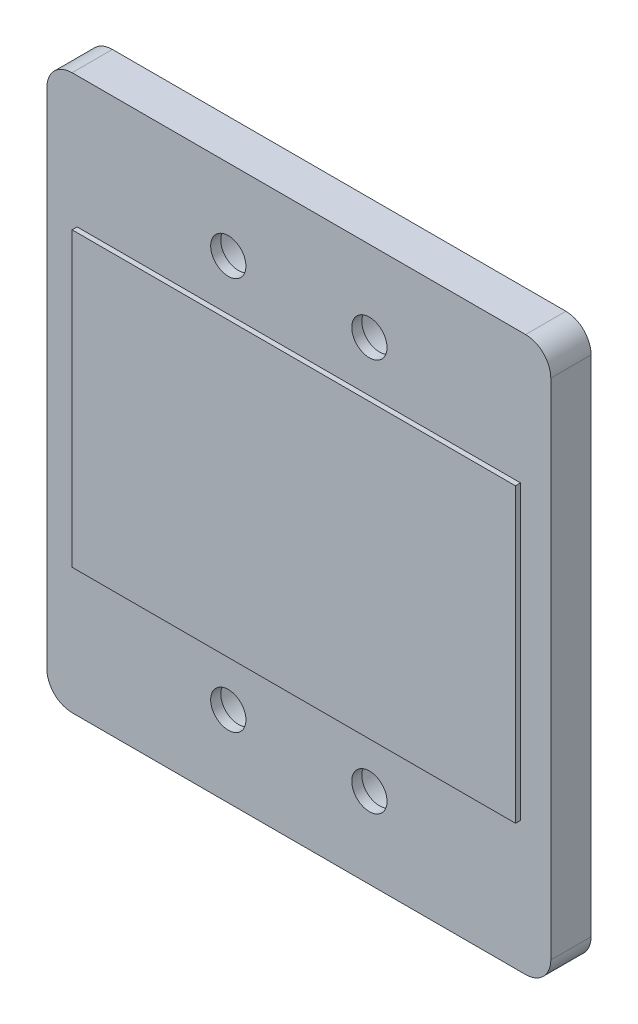
from build123d import *

# Parameters (mm, degrees)
BOSS_EXTRUDE1_DEPTH = 8
SKETCH2_W           = 88
SKETCH2_H           = 58
BOSS_EXTRUDE2_DEPTH = 1
SKETCH4_R           = 6
CUT_EXTRUDE1_DEPTH  = 6
SKETCH5_R           = 3.5
CUT_EXTRUDE2_DEPTH  = 6


with BuildPart() as part:
    # Sketch1 → Boss-Extrude1 (new body)
    with BuildSketch(Plane.XY):
        with BuildLine():
            Line((-45, -55), (45, -55))
            ThreePointArc((45, -55), (48.535533906, -53.535533906), (50, -50))
            Line((50, -50), (50, 50))
            ThreePointArc((50, 50), (48.535533906, 53.535533906), (45, 55))
            Line((45, 55), (-45, 55))
            ThreePointArc((-45, 55), (-48.535533906, 53.535533906), (-50, 50))
            Line((-50, 50), (-50, -50))
            ThreePointArc((-50, -50), (-48.535533906, -53.535533906), (-45, -55))
        make_face()
    extrude(amount=BOSS_EXTRUDE1_DEPTH)

    # Sketch2 → Boss-Extrude2 (add)
    with BuildSketch(Plane.XY.offset(8)):
        Rectangle(SKETCH2_W, SKETCH2_H)
    extrude(amount=BOSS_EXTRUDE2_DEPTH)

    # Sketch4 → Cut-Extrude1 (cut)
    with BuildSketch(Plane(origin=(0, 0, 0), x_dir=(-1, 0, 0), z_dir=(0, 0, -1))):
        with Locations((-14, -39)):
            Circle(SKETCH4_R)
        with Locations((14, -39)):
            Circle(SKETCH4_R)
        with Locations(Location((14, 39, 0), (0, 0, 180))):
            Circle(SKETCH4_R)
        with Locations(Location((-14, 39, 0), (0, 0, 180))):
            Circle(SKETCH4_R)
    extrude(amount=-CUT_EXTRUDE1_DEPTH, mode=Mode.SUBTRACT)

    # Sketch5 → Cut-Extrude2 (cut)
    with BuildSketch(Plane(origin=(0, 0, 6), x_dir=(-1, 0, 0), z_dir=(0, 0, -1))):
        with Locations((-14, 39)):
            Circle(SKETCH5_R)
        with Locations((14, 39)):
            Circle(SKETCH5_R)
        with Locations((14, -39)):
            Circle(SKETCH5_R)
        with Locations((-14, -39)):
            Circle(SKETCH5_R)
    extrude(amount=-CUT_EXTRUDE2_DEPTH, mode=Mode.SUBTRACT)


solid = part.part
